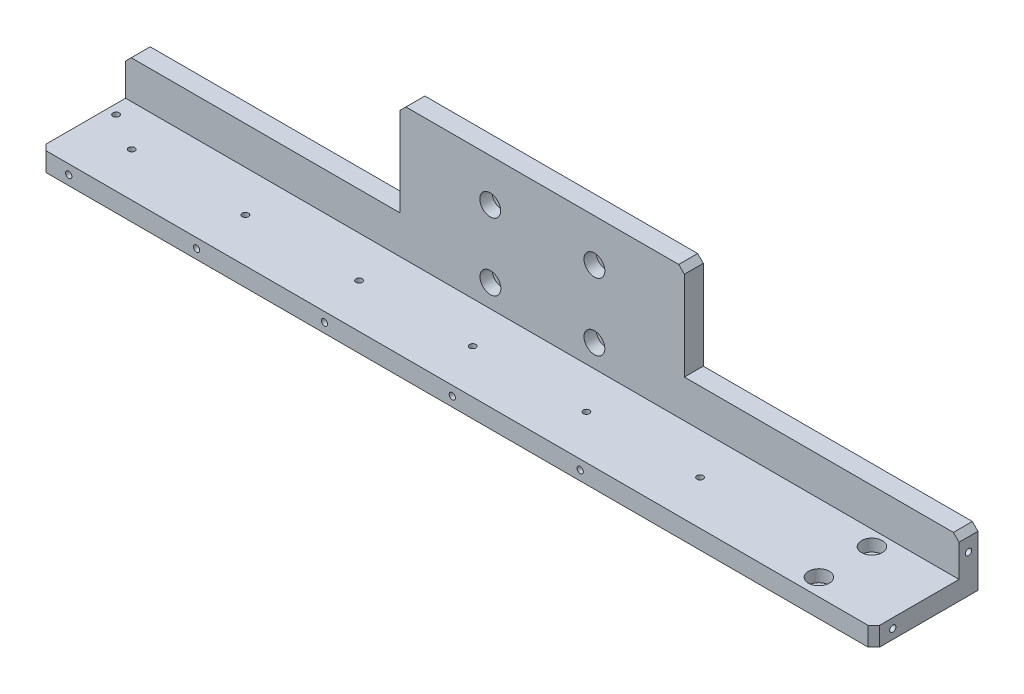
from build123d import *

# Parameters (mm, degrees)
SKETCH_2_W                   = 440
SKETCH_2_H                   = 80
EXTRUDE_1_DEPTH              = 10
SKETCH_3_W                   = 440
SKETCH_3_H                   = 10
EXTRUDE_2_DEPTH              = 45
SKETCH_5_W                   = 145
SKETCH_5_H                   = 50
CUT_EXTRUDE_2_DEPTH          = 239.379948821
HOLE_WIZARD_M6_1_D           = 6.6
HOLE_WIZARD_M6_1_DEPTH       = 22.25
HOLE_WIZARD_M6_1_CBORE_D     = 11
HOLE_WIZARD_M6_1_CBORE_DEPTH = 6.4
HOLE_WIZARD_M6_1_TIP         = 1.982840043
HOLE_WIZARD_M4_1_D           = 3.3
HOLE_WIZARD_M4_1_DEPTH       = 11.5
HOLE_WIZARD_M4_1_TIP         = 0.991420021
HOLE_WIZARD_M4_2_D           = 3.3
HOLE_WIZARD_M4_2_DEPTH       = 11.5
HOLE_WIZARD_M4_2_TIP         = 0.991420021
CHAMFER_1_SIZE               = 3
HOLE_WIZARD_M6_2_D           = 6.6
HOLE_WIZARD_M6_2_DEPTH       = 17
HOLE_WIZARD_M6_2_CBORE_D     = 11
HOLE_WIZARD_M6_2_CBORE_DEPTH = 6.4
HOLE_WIZARD_M6_2_TIP         = 1.982840043
HOLE_WIZARD_M4_3_D           = 3.3
HOLE_WIZARD_M4_3_DEPTH       = 11.5
HOLE_WIZARD_M4_3_TIP         = 0.991420021
HOLE_WIZARD_M4_4_AT_2_COUNT  = 2
HOLE_WIZARD_M4_4_AT_2_PITCH  = 42.720018727
HOLE_WIZARD_M4_5_D           = 3.3
HOLE_WIZARD_M4_5_DEPTH       = 11.5
HOLE_WIZARD_M4_5_TIP         = 0.991420021


with BuildPart() as part:
    # 草图2 → 凸台-拉伸1 (new body)
    with BuildSketch(Plane.XY):
        with Locations((0, -40)):
            Rectangle(SKETCH_2_W, SKETCH_2_H)
    extrude(amount=EXTRUDE_1_DEPTH)

    # 草图3 → 凸台-拉伸2 (add)
    with BuildSketch(Plane.XY.offset(10)):
        with Locations((0, -75)):
            Rectangle(SKETCH_3_W, SKETCH_3_H)
    extrude(amount=EXTRUDE_2_DEPTH)

    # 草图5 → 切除-拉伸2 (cut, through all)
    with BuildSketch(Plane.XY.offset(10)):
        with Locations((-147.5, -25)):
            Rectangle(SKETCH_5_W, SKETCH_5_H)
        with Locations((147.5, -25)):
            Rectangle(SKETCH_5_W, SKETCH_5_H)
    extrude(amount=-CUT_EXTRUDE_2_DEPTH, mode=Mode.SUBTRACT)

    # M6 六角凹头螺钉的柱形沉头孔1
    with Locations(Plane.XY.offset(10)):
        with Locations((-27.5, -22.520483068), (27.5, -22.520483068), (27.5, -58), (-27.396175046, -58)):
            CounterBoreHole(HOLE_WIZARD_M6_1_D / 2, HOLE_WIZARD_M6_1_CBORE_D / 2, HOLE_WIZARD_M6_1_CBORE_DEPTH, depth=HOLE_WIZARD_M6_1_DEPTH)
            with Locations((0, 0, -(HOLE_WIZARD_M6_1_DEPTH + HOLE_WIZARD_M6_1_TIP / 2))):  # 118° drill point
                Cone(0, HOLE_WIZARD_M6_1_D / 2, HOLE_WIZARD_M6_1_TIP, mode=Mode.SUBTRACT)

    # M4 螺纹孔1
    with Locations(Plane(origin=(0, -70, 0), x_dir=(1, 0, 0), z_dir=(0, 1, 0))):
        with Locations((-195, -31.742753413), (-135, -31.742753413), (-75, -31.742753413), (-15, -31.742753413), (45, -31.742753413), (105, -31.742753413)):
            Hole(HOLE_WIZARD_M4_1_D / 2, depth=HOLE_WIZARD_M4_1_DEPTH)
            with Locations((0, 0, -(HOLE_WIZARD_M4_1_DEPTH + HOLE_WIZARD_M4_1_TIP / 2))):  # 118° drill point
                Cone(0, HOLE_WIZARD_M4_1_D / 2, HOLE_WIZARD_M4_1_TIP, mode=Mode.SUBTRACT)

    # M4 螺纹孔2
    with Locations(Plane.XY.offset(55)):
        with Locations((-205, -75), (-137.5, -75), (-70, -75), (-2.5, -75), (65, -75)):
            Hole(HOLE_WIZARD_M4_2_D / 2, depth=HOLE_WIZARD_M4_2_DEPTH)
            with Locations((0, 0, -(HOLE_WIZARD_M4_2_DEPTH + HOLE_WIZARD_M4_2_TIP / 2))):  # 118° drill point
                Cone(0, HOLE_WIZARD_M4_2_D / 2, HOLE_WIZARD_M4_2_TIP, mode=Mode.SUBTRACT)

    # 倒角1
    chamfer_1_edges = [part.edges().sort_by_distance(p)[0] for p in [
        (-220, -75, 55),
        (220, -75, 55),
        (-220, -50, 5),
        (-75, 0, 5),
        (75, 0, 5),
        (220, -50, 5),
    ]]
    chamfer(chamfer_1_edges, length=CHAMFER_1_SIZE)

    # M6 六角凹头螺钉的柱形沉头孔2
    with Locations(Plane(origin=(0, -70, 0), x_dir=(1, 0, 0), z_dir=(0, 1, 0))):
        with Locations((182, -18), (182, -46)):
            CounterBoreHole(HOLE_WIZARD_M6_2_D / 2, HOLE_WIZARD_M6_2_CBORE_D / 2, HOLE_WIZARD_M6_2_CBORE_DEPTH, depth=HOLE_WIZARD_M6_2_DEPTH)
            with Locations((0, 0, -(HOLE_WIZARD_M6_2_DEPTH + HOLE_WIZARD_M6_2_TIP / 2))):  # 118° drill point
                Cone(0, HOLE_WIZARD_M6_2_D / 2, HOLE_WIZARD_M6_2_TIP, mode=Mode.SUBTRACT)

    # M4 螺纹孔3
    with Locations(Plane(origin=(0, -70, 0), x_dir=(1, 0, 0), z_dir=(0, 1, 0))):
        with Locations((-215, -20)):
            Hole(HOLE_WIZARD_M4_3_D / 2, depth=HOLE_WIZARD_M4_3_DEPTH)
            with Locations((0, 0, -(HOLE_WIZARD_M4_3_DEPTH + HOLE_WIZARD_M4_3_TIP / 2))):  # 118° drill point
                Cone(0, HOLE_WIZARD_M4_3_D / 2, HOLE_WIZARD_M4_3_TIP, mode=Mode.SUBTRACT)

    # 草图17 → M4 螺纹孔4 (revolve, cut)
    with BuildSketch(Plane(origin=(-220, -75, 45), x_dir=(0, 0, 1), z_dir=(0, 1, 0))):
        Polygon((0, 0), (0, 12.491420021), (1.65, 11.5), (1.65, 0), align=None)
    hole_wizard_m4_4 = revolve(axis=Axis((-226.35, -75, 45), (1, 0, 0)), mode=Mode.SUBTRACT)

    # M4 螺纹孔4 at 2: M4 螺纹孔4 ×2
    with Locations(*[Vector(0, 0.35112344158839187, -0.9363291775690445) * (i * HOLE_WIZARD_M4_4_AT_2_PITCH) for i in range(1, HOLE_WIZARD_M4_4_AT_2_COUNT)]):
        add(hole_wizard_m4_4, mode=Mode.SUBTRACT)

    # 镜向1: M4 螺纹孔4 across plane
    add(hole_wizard_m4_4.mirror(Plane(origin=(0, 0, 0), x_dir=(0, 0, 1), z_dir=(1, 0, 0))), mode=Mode.SUBTRACT)

    # 镜向1 copy 1 sketch → 镜向1 copy 1 (revolve, cut)
    with BuildSketch(Plane(origin=(220, -60, 5), x_dir=(0, 0, 1), z_dir=(0, 1, 0))):
        Polygon((0, 0), (0, -12.491420021), (1.65, -11.5), (1.65, 0), align=None)
    revolve(axis=Axis((226.35, -60, 5), (1, 0, 0)), mode=Mode.SUBTRACT)

    # M4 螺纹孔5
    with Locations(Plane(origin=(0, 0, 0), x_dir=(-1, 0, 0), z_dir=(0, 0, -1))):
        with Locations((-47.5, -75), (47.5, -75)):
            Hole(HOLE_WIZARD_M4_5_D / 2, depth=HOLE_WIZARD_M4_5_DEPTH)
            with Locations((0, 0, -(HOLE_WIZARD_M4_5_DEPTH + HOLE_WIZARD_M4_5_TIP / 2))):  # 118° drill point
                Cone(0, HOLE_WIZARD_M4_5_D / 2, HOLE_WIZARD_M4_5_TIP, mode=Mode.SUBTRACT)


solid = part.part
